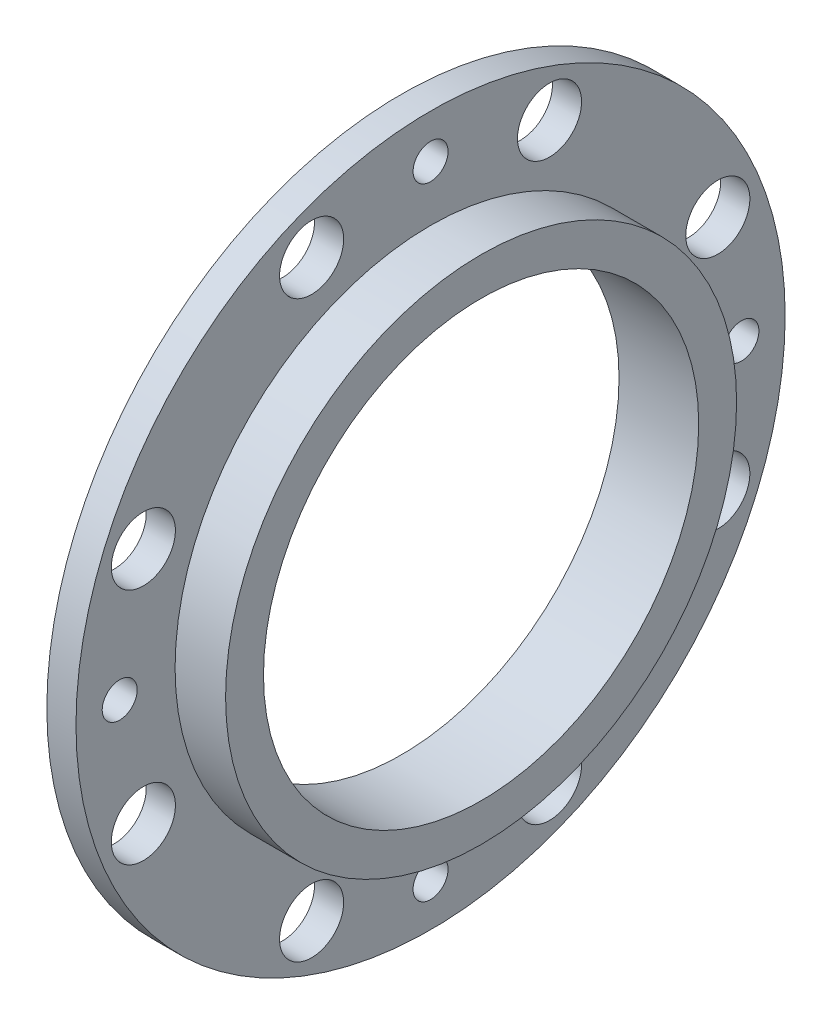
from build123d import *

# Parameters (mm, degrees)
SKETCH2_R          = 16.5
CUT_EXTRUDE1_DEPTH = 20
SKETCH3_R          = 9
CUT_EXTRUDE2_DEPTH = 20


with BuildPart() as part:
    # Sketch1 → Revolve1 (revolve)
    with BuildSketch(Plane.XY, mode=Mode.PRIVATE) as revolve1_sk:
        Polygon((-19.588974855, 112), (-19.588974855, 182.5), (-4.588974855, 182.5), (-4.588974855, 131.5), (21.411025145, 131.5), (21.411025145, 112), align=None)
    revolve(revolve1_sk.sketch.rotate(Axis((-91.426499033, 0, 0), (1, 0, 0)), 90), axis=Axis((-91.426499033, 0, 0), (1, 0, 0)))

    # Sketch2 → Cut-Extrude1 (cut)
    with BuildSketch(Plane.ZY.offset(19.588974855)):
        with Locations((61.229349178, 147.820725202)):
            Circle(SKETCH2_R)
        with Locations((147.820725202, 61.229349178)):
            Circle(SKETCH2_R)
        with Locations((147.820725202, -61.229349178)):
            Circle(SKETCH2_R)
        with Locations((61.229349178, -147.820725202)):
            Circle(SKETCH2_R)
        with Locations((-61.229349178, -147.820725202)):
            Circle(SKETCH2_R)
        with Locations((-147.820725202, -61.229349178)):
            Circle(SKETCH2_R)
        with Locations((-147.820725202, 61.229349178)):
            Circle(SKETCH2_R)
        with Locations((-61.229349178, 147.820725202)):
            Circle(SKETCH2_R)
    extrude(amount=-CUT_EXTRUDE1_DEPTH, mode=Mode.SUBTRACT)

    # Sketch3 → Cut-Extrude2 (cut)
    with BuildSketch(Plane.ZY.offset(19.588974855)):
        with Locations((0, 160)):
            Circle(SKETCH3_R)
        with Locations((160, 0)):
            Circle(SKETCH3_R)
        with Locations((0, -160)):
            Circle(SKETCH3_R)
        with Locations((-160, 0)):
            Circle(SKETCH3_R)
    extrude(amount=-CUT_EXTRUDE2_DEPTH, mode=Mode.SUBTRACT)


solid = part.part
